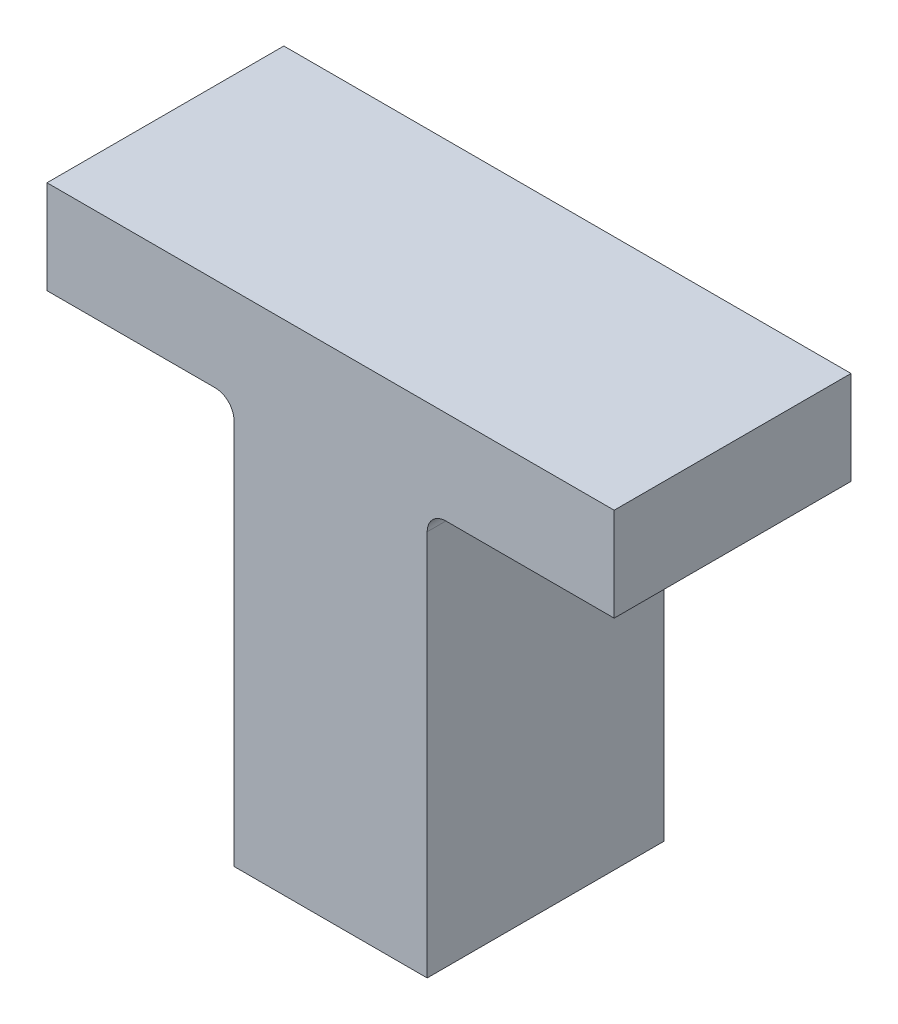
from build123d import *

# Parameters (mm, degrees)
SKETCH_1_W          = 91
SKETCH_1_H          = 80
EXTRUDE_1_DEPTH     = 19
CUT_EXTRUDE_1_REACH = 73.514
SKETCH_2_W          = 30
SKETCH_2_H          = 65
FILLET_1_R          = 3


with BuildPart() as part:
    # 草图1 → 凸台-拉伸1 (new, symmetric)
    with BuildSketch(Plane.XY):
        Rectangle(SKETCH_1_W, SKETCH_1_H)
    extrude(amount=EXTRUDE_1_DEPTH, both=True)

    # 草图2 → 切除-拉伸1 (cut, up to next)
    with BuildSketch(Plane.XY.offset(19), mode=Mode.PRIVATE) as cut_extrude_1_sk1:
        with Locations((-30.5, -7.5)):
            Rectangle(SKETCH_2_W, SKETCH_2_H)
    cut_extrude_1_tool1 = extrude(cut_extrude_1_sk1.sketch, amount=-CUT_EXTRUDE_1_REACH, mode=Mode.PRIVATE) & part.part
    # 草图2 → 切除-拉伸1 (cut, up to next)
    with BuildSketch(Plane.XY.offset(19), mode=Mode.PRIVATE) as cut_extrude_1_sk2:
        with Locations((30.5, -7.5)):
            Rectangle(SKETCH_2_W, SKETCH_2_H)
    cut_extrude_1_tool2 = extrude(cut_extrude_1_sk2.sketch, amount=-CUT_EXTRUDE_1_REACH, mode=Mode.PRIVATE) & part.part
    add(cut_extrude_1_tool1.solids().sort_by_distance((-30.5, -7.5, 19))[0], mode=Mode.SUBTRACT)
    add(cut_extrude_1_tool2.solids().sort_by_distance((30.5, -7.5, 19))[0], mode=Mode.SUBTRACT)

    # 圆角1
    fillet_1_edges = [part.edges().sort_by_distance(p)[0] for p in [
        (-15.5, 25, 0),
        (15.5, 25, 0),
    ]]
    fillet(fillet_1_edges, radius=FILLET_1_R)


solid = part.part
